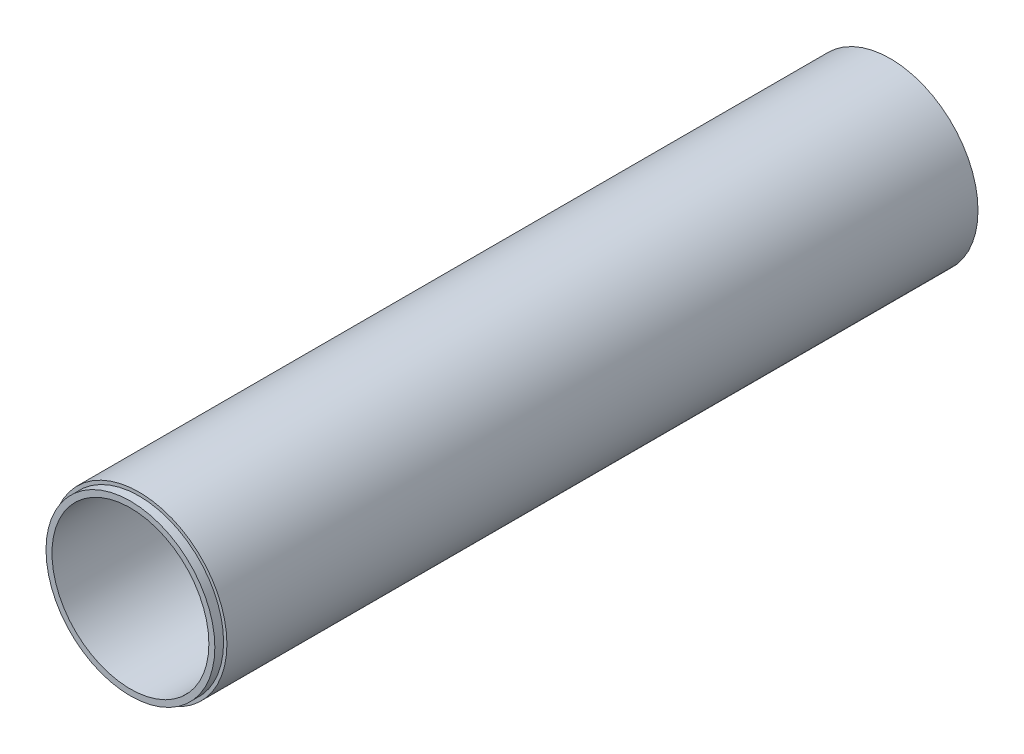
SolidWorks part; units mm, degrees
material "1023 碳钢板 (SS)"
ref_plane "前视基准面" through (0, 0, 0) normal (0, 0, 1) x (1, 0, 0)
ref_plane "上视基准面" through (0, 0, 0) normal (0, 1, 0) x (1, 0, 0)
ref_plane "右视基准面" through (0, 0, 0) normal (1, 0, 0) x (0, 0, -1)
sketch "草图1" plane through (0, 0, 0) normal (0, 0, 1) x (1, 0, 0)
  circle A0 centre (0, 0) radius 30.15
  dimension "D1" = 60.3
extrude "凸台-拉伸1" add sketch "草图1" along normal blind 261
shell "抽壳1" thickness 3.2
sketch "草图2" plane through (0, 0, 261) normal (0, 0, 1) x (1, 0, 0)
  circle A0 centre (0, 0) radius 29
  dimension "D1" = 58
extrude "切除-拉伸1" cut sketch "草图2" against normal blind 3 flip side to cut
